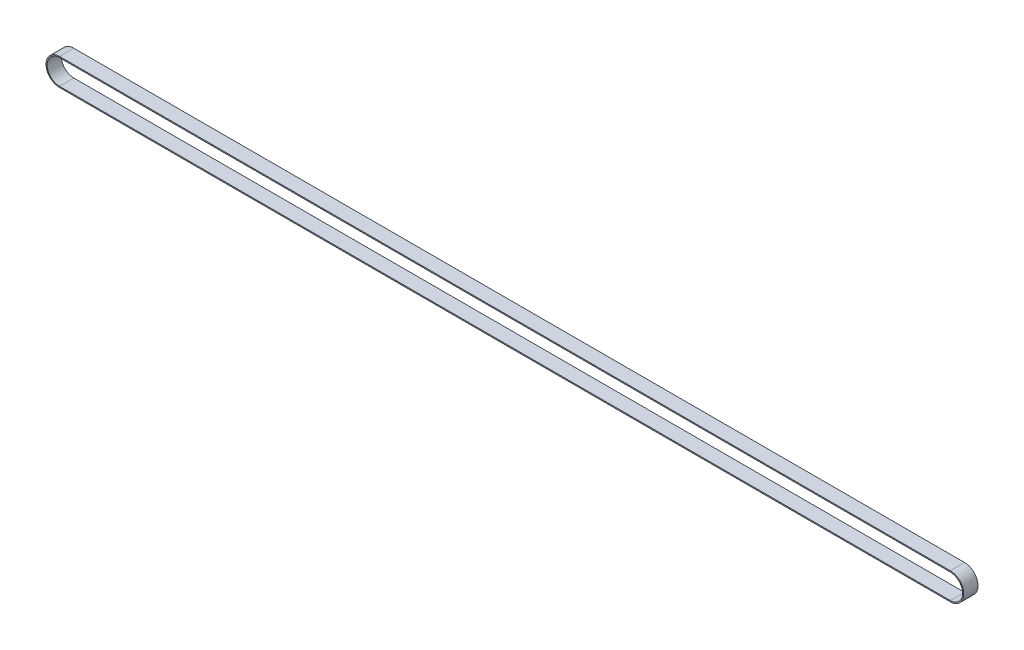
SolidWorks part; units mm, degrees
material "6061 合金"
ref_plane "前视基准面" through (0, 0, 0) normal (0, 0, 1) x (1, 0, 0)
ref_plane "上视基准面" through (0, 0, 0) normal (0, 1, 0) x (1, 0, 0)
ref_plane "右视基准面" through (0, 0, 0) normal (1, 0, 0) x (0, 0, -1)
sketch "草图1" plane through (0, 0, 0) normal (0, 0, 1) x (1, 0, 0)
  line L0 (0, 12.99) -> (937, 12.99)
  line L1 (937, -12.99) -> (0, -12.99)
  line L2 (0, 14.17) -> (937, 14.17)
  line L3 (937, -14.17) -> (0, -14.17)
  arc A0 (0, 12.99) -> (0, -12.99) centre (0, 0) ccw
  arc A1 (937, -12.99) -> (937, 12.99) centre (937, 0) ccw
  arc A2 (937, -14.17) -> (937, 14.17) centre (937, 0) ccw
  arc A3 (0, 14.17) -> (0, -14.17) centre (0, 0) ccw
  dimension "D1" = 25.98
  dimension "D2" = 25.98
  dimension "D3" = 937
  dimension "D4" = 1.18
extrude "凸台-拉伸1" add sketch "草图1" along normal mid plane 15
